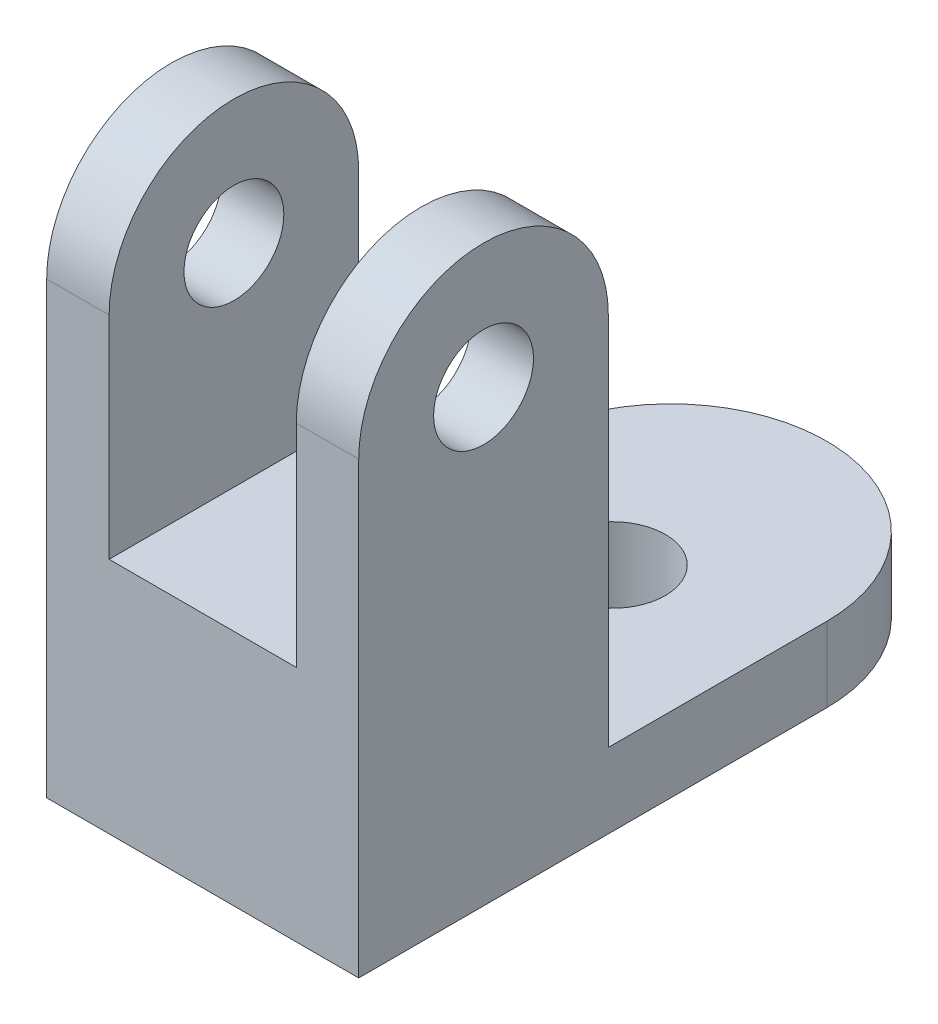
from build123d import *

# Parameters (mm, degrees)
SKETCH1_W           = 25
SKETCH1_H           = 50
BOSS_EXTRUDE1_DEPTH = 6
SKETCH2_W           = 25
SKETCH2_H           = 20
BOSS_EXTRUDE2_DEPTH = 40
FILLET1_RADIUS      = 12.5
FILLET1_LENGTH      = 6
FILLET3_RADIUS      = 10
FILLET3_LENGTH      = 25
CUT_EXTRUDE1_START  = -5
SKETCH3_W           = 21.31771447
SKETCH3_H           = 40.676557725
CUT_EXTRUDE1_DEPTH  = 15
SKETCH4_R           = 4
CUT_EXTRUDE2_DEPTH  = 59.017238817
SKETCH5_R           = 4.25
CUT_EXTRUDE3_DEPTH  = 49.79805324


with BuildPart() as part:
    # Sketch1 → Boss-Extrude1 (new body)
    with BuildSketch(Plane(origin=(0, 0, 0), x_dir=(1, 0, 0), z_dir=(0, 1, 0))):
        Rectangle(SKETCH1_W, SKETCH1_H)
    extrude(amount=BOSS_EXTRUDE1_DEPTH)

    # Sketch2 → Boss-Extrude2 (add)
    with BuildSketch(Plane(origin=(0, 6, 0), x_dir=(1, 0, 0), z_dir=(0, 1, 0))):
        with Locations((0, -15)):
            Rectangle(SKETCH2_W, SKETCH2_H)
    extrude(amount=BOSS_EXTRUDE2_DEPTH)

    # Fillet1: full round fillet: the end face becomes a half cylinder, R = half its width
    fillet1_face = Plane((0, 3, -25), x_dir=(0, 1, 0), z_dir=(0, 0, -1))  # on the end face: x along it, z out of the body
    fillet1_slab = fillet1_face.offset(-FILLET1_RADIUS / 2) * Box(FILLET1_LENGTH, 2 * FILLET1_RADIUS, FILLET1_RADIUS, mode=Mode.PRIVATE)  # the body's end, R deep
    fillet1_round = Plane((0, 3, -12.5), x_dir=(0, 0, -1), z_dir=(0, 1, 0)) * Cylinder(FILLET1_RADIUS, FILLET1_LENGTH, mode=Mode.PRIVATE)  # its axis R under the face
    add(fillet1_slab - fillet1_round, mode=Mode.SUBTRACT)

    # Fillet3: full round fillet: the end face becomes a half cylinder, R = half its width
    fillet3_face = Plane((0, 46, 15), x_dir=(-1, 0, 0), z_dir=(0, 1, 0))  # on the end face: x along it, z out of the body
    fillet3_slab = fillet3_face.offset(-FILLET3_RADIUS / 2) * Box(FILLET3_LENGTH, 2 * FILLET3_RADIUS, FILLET3_RADIUS, mode=Mode.PRIVATE)  # the body's end, R deep
    fillet3_round = Plane((0, 36, 15), x_dir=(0, 1, 0), z_dir=(-1, 0, 0)) * Cylinder(FILLET3_RADIUS, FILLET3_LENGTH, mode=Mode.PRIVATE)  # its axis R under the face
    add(fillet3_slab - fillet3_round, mode=Mode.SUBTRACT)

    # Sketch3 → Cut-Extrude1 (cut)
    with BuildSketch(Plane.ZY.offset(12.5).offset(CUT_EXTRUDE1_START)):
        with Locations((15.658857235, 39.391263894)):
            Rectangle(SKETCH3_W, SKETCH3_H)
    extrude(amount=-CUT_EXTRUDE1_DEPTH, mode=Mode.SUBTRACT)

    # Sketch4 → Cut-Extrude2 (cut, through all)
    with BuildSketch(Plane.ZY.offset(12.5)):
        with Locations((15, 36)):
            Circle(SKETCH4_R)
    extrude(amount=-CUT_EXTRUDE2_DEPTH, mode=Mode.SUBTRACT)

    # Sketch5 → Cut-Extrude3 (cut, through all)
    with BuildSketch(Plane(origin=(0, 6, 0), x_dir=(1, 0, 0), z_dir=(0, 1, 0))):
        with Locations(Location((0, 7.814758418, 0), (0, 0, 270))):
            Circle(SKETCH5_R)
    extrude(amount=-CUT_EXTRUDE3_DEPTH, mode=Mode.SUBTRACT)


solid = part.part
